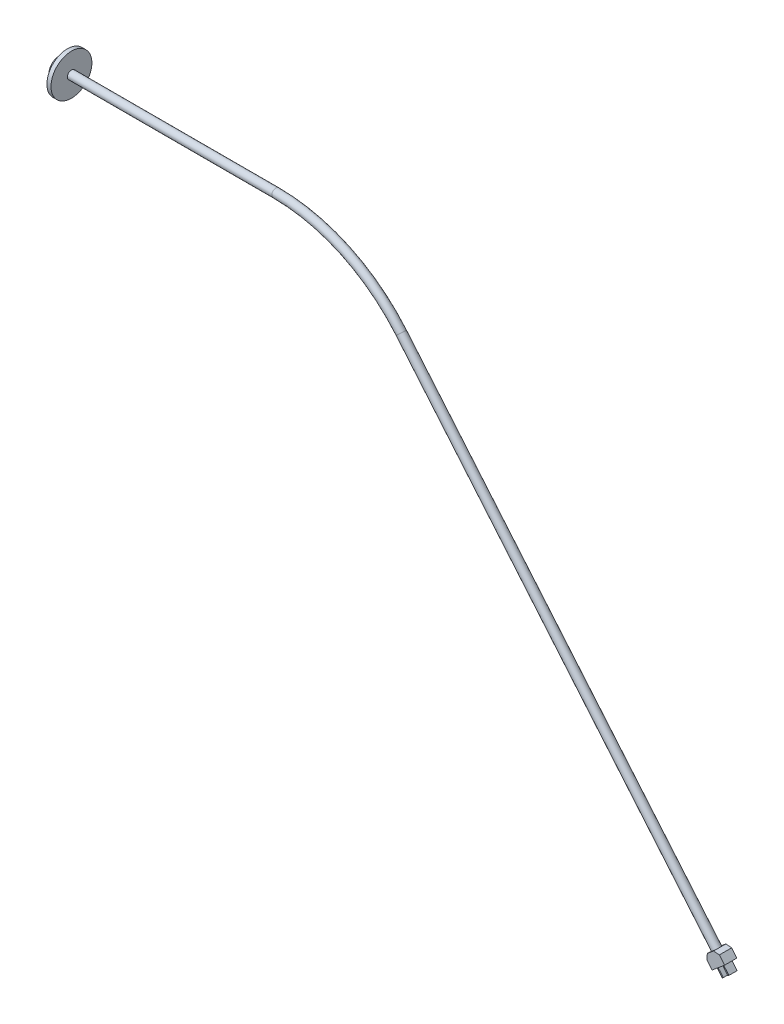
from build123d import *

# Parameters (mm, degrees)
SWEEP1_PROFILE_R    = 1
BOSS_EXTRUDE1_DEPTH = 1.5
BOSS_EXTRUDE2_DEPTH = 1


with BuildPart() as part:
    # Sketch1 → Revolve1 (revolve)
    with BuildSketch(Plane.XY, mode=Mode.PRIVATE) as revolve1_sk:
        Polygon((0, 0), (0, 2.5), (2, 2.5), (2, 5), (3, 5), (3, 0), align=None)
    revolve(revolve1_sk.sketch.rotate(Axis((0, 0, 0), (1, 0, 0)), 90), axis=Axis((0, 0, 0), (1, 0, 0)))

    # Sweep1: sweep along a path in Sketch2
    with BuildLine(Plane.XY) as sweep1_path:
        Line((3, 0), (53, 0))
        ThreePointArc((53, 0), (69.90473047, -3.747688519), (83.641777725, -14.288495613))
        Line((83.641777725, -14.288495613), (160.776290887, -106.213828787))
    # Sweep1 profile (on start of the path) → Sweep1 (sweep)
    with BuildSketch(Plane(origin=(3, 0, 0), x_dir=(0, 0, 1), z_dir=(1, 0, 0))):
        Circle(SWEEP1_PROFILE_R)
    sweep(path=sweep1_path.line)

    # Sketch11 → Boss-Extrude1 (add, symmetric)
    with BuildSketch(Plane.XY):
        Polygon((160.010246444, -106.856616397), (161.54233533, -105.571041177), (162.951167383, -105.694298011), (164.236742602, -107.226386897), (161.17256483, -109.797537336), (159.886989611, -108.265448449), align=None)
    extrude(amount=BOSS_EXTRUDE1_DEPTH, both=True)

    # Sketch12 → Boss-Extrude2 (add, symmetric)
    with BuildSketch(Plane.XY):
        Polygon((163.509000381, -107.837035126), (164.794575601, -109.369124012), (164.564762268, -109.561960295), (163.279187049, -108.029871409), align=None)
        Polygon((162.130120384, -108.994052823), (161.900307051, -109.186889106), (163.18588227, -110.718977993), (163.415695603, -110.52614171), align=None)
    extrude(amount=BOSS_EXTRUDE2_DEPTH, both=True)


solid = part.part
